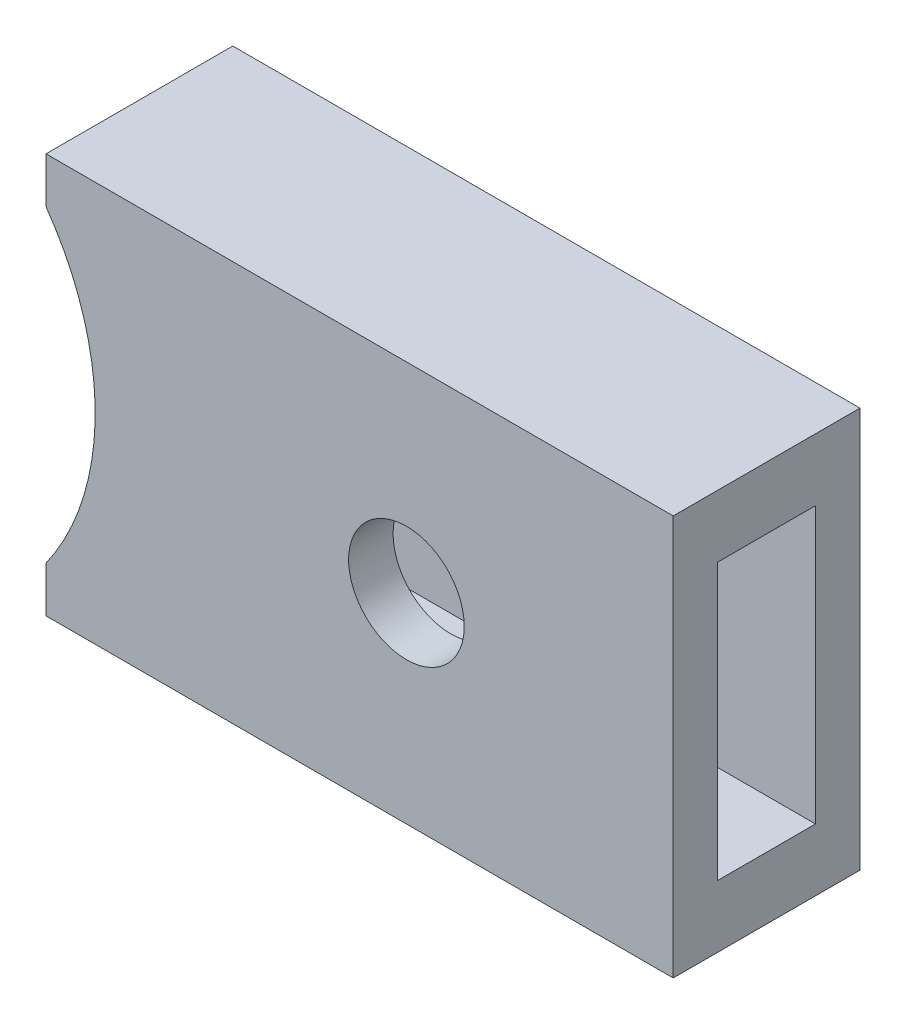
from build123d import *

# Parameters (mm, degrees)
EXTRUDE_1_DEPTH     = 10.5
SKETCH_2_W          = 11
SKETCH_2_H          = 31
CUT_EXTRUDE_1_DEPTH = 75.76938691
CUT_EXTRUDE_2_REACH = 101.861
SKETCH_3_R          = 6.5
CUT_EXTRUDE_5_REACH = 101.861
SKETCH_4_R          = 6.5


with BuildPart() as part:
    # 草图1 → 凸台-拉伸1 (new, symmetric)
    with BuildSketch(Plane.XY):
        with BuildLine():
            Line((95, 22.5), (95, -22.5))
            Line((95, -22.5), (24.473684211, -22.5))
            Line((24.473684211, -22.5), (24.473684211, -17.350469191))
            ThreePointArc((24.473684211, -17.350469191), (30, 0), (24.473684211, 17.350469191))
            Line((24.473684211, 17.350469191), (24.473684211, 22.5))
            Line((24.473684211, 22.5), (95, 22.5))
        make_face()
    extrude(amount=EXTRUDE_1_DEPTH, both=True)

    # 草图2 → 切除-拉伸1 (cut, through all)
    with BuildSketch(Plane(origin=(95, 0, 0), x_dir=(0, 0, -1), z_dir=(1, 0, 0))):
        Rectangle(SKETCH_2_W, SKETCH_2_H)
    extrude(amount=-CUT_EXTRUDE_1_DEPTH, mode=Mode.SUBTRACT)

    # 草图3 → 切除-拉伸2 (cut, up to next)
    with BuildSketch(Plane.XY.offset(10.5), mode=Mode.PRIVATE) as cut_extrude_2_sk1:
        with Locations((65, 0)):
            Circle(SKETCH_3_R)
    cut_extrude_2_tool1 = extrude(cut_extrude_2_sk1.sketch, amount=-CUT_EXTRUDE_2_REACH, mode=Mode.PRIVATE) & part.part
    add(cut_extrude_2_tool1.solids().sort_by_distance((65, 0, 10.5))[0], mode=Mode.SUBTRACT)

    # 草图4 → 切除-拉伸5 (cut, up to next)
    with BuildSketch(Plane(origin=(0, 0, -10.5), x_dir=(-1, 0, 0), z_dir=(0, 0, -1)), mode=Mode.PRIVATE) as cut_extrude_5_sk1:
        Polygon((-76.55, 0), (-70.779489597, -10), (-59.220510403, -10), (-53.45, 0), (-59.220510403, 10), (-70.779489597, 10), align=None)
        with Locations(Location((-65, 0, 0), (0, 0, 180))):
            Circle(SKETCH_4_R, mode=Mode.SUBTRACT)
    cut_extrude_5_tool1 = extrude(cut_extrude_5_sk1.sketch, amount=-CUT_EXTRUDE_5_REACH, mode=Mode.PRIVATE) & part.part
    # 草图4 → 切除-拉伸5 (cut, up to next)
    with BuildSketch(Plane(origin=(0, 0, -10.5), x_dir=(-1, 0, 0), z_dir=(0, 0, -1)), mode=Mode.PRIVATE) as cut_extrude_5_sk2:
        with Locations(Location((-65, 0, 0), (0, 0, 180))):
            Circle(SKETCH_4_R)
    cut_extrude_5_tool2 = extrude(cut_extrude_5_sk2.sketch, amount=-CUT_EXTRUDE_5_REACH, mode=Mode.PRIVATE) & part.part
    add(cut_extrude_5_tool1.solids().sort_by_distance((73.400096, -4.847284, -10.5))[0], mode=Mode.SUBTRACT)
    add(cut_extrude_5_tool2.solids().sort_by_distance((65, 0, -10.5))[0], mode=Mode.SUBTRACT)


solid = part.part
